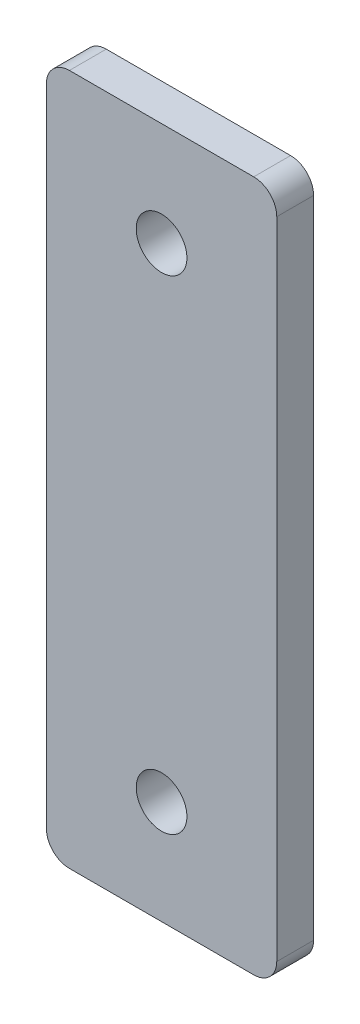
from build123d import *

# Parameters (mm, degrees)
BOSS_EXTRUDE1_DEPTH        = 8
F_11_0_11_DIAMETER_HOLE5_D = 11


with BuildPart() as part:
    # Sketch1 → Boss-Extrude1 (new body)
    with BuildSketch(Plane.XY):
        with BuildLine():
            Line((20, -75), (-20, -75))
            ThreePointArc((-20, -75), (-23.535533906, -73.535533906), (-25, -70))
            Line((-25, -70), (-25, 70))
            ThreePointArc((-25, 70), (-23.535533906, 73.535533906), (-20, 75))
            Line((-20, 75), (20, 75))
            ThreePointArc((20, 75), (23.535533906, 73.535533906), (25, 70))
            Line((25, 70), (25, -70))
            ThreePointArc((25, -70), (23.535533906, -73.535533906), (20, -75))
        make_face()
    extrude(amount=BOSS_EXTRUDE1_DEPTH)

    # Ø11.0 (11) Diameter Hole5 (through all)
    with Locations(Plane.XY.offset(8)):
        with Locations((0, 52.5), (0, -52.5)):
            Hole(F_11_0_11_DIAMETER_HOLE5_D / 2)


solid = part.part
